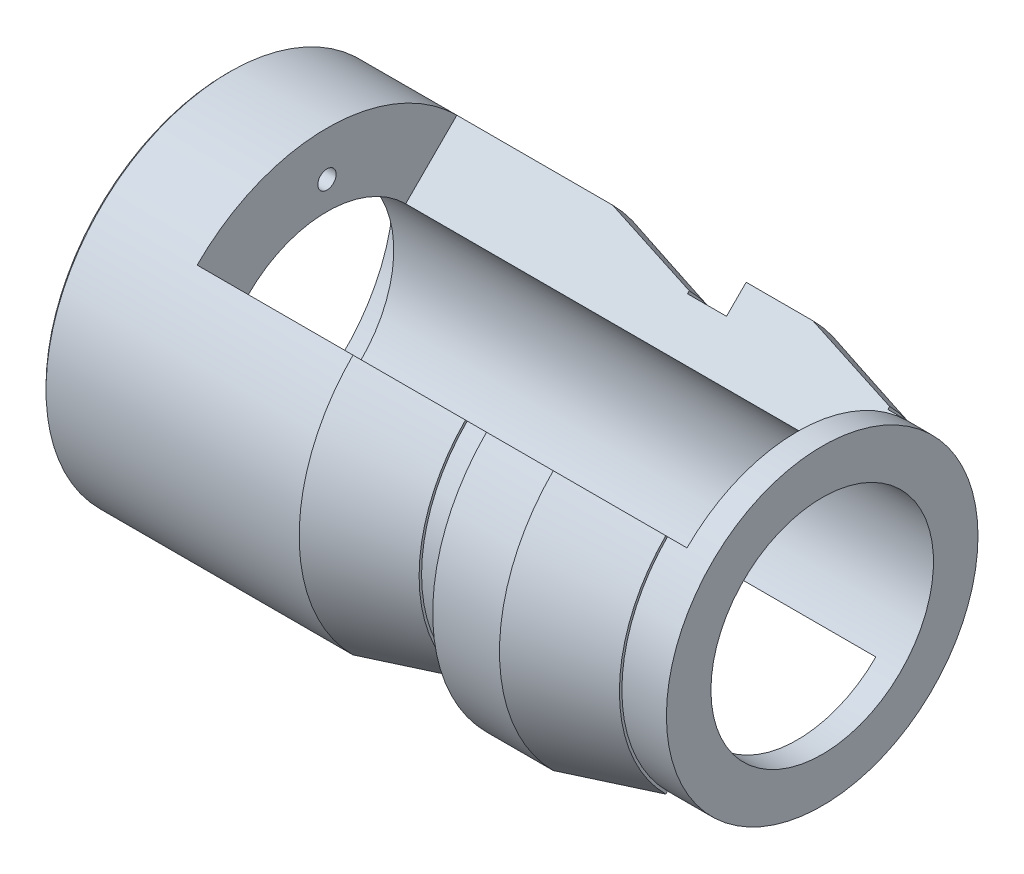
from build123d import *

# Parameters (mm, degrees)
CUT_REVOLVE_1_ANGLE    = 90
CHAMFER_1_SIZE         = 0.5
HOLE_WIZARD_M4_1_D     = 3.3
HOLE_WIZARD_M4_1_DEPTH = 11.5
HOLE_WIZARD_M4_1_TIP   = 0.991420021


with BuildPart() as part:
    # 草图1 → 旋转1 (revolve)
    with BuildSketch(Plane.XY, mode=Mode.PRIVATE) as revolve_1_sk:
        Polygon((0, 30), (10, 30), (10, 20), (107, 20), (107, 28), (99, 28), (99, 28.444863729), (82, 33), (70, 33), (70, 28), (63, 28), (63, 28.444863729), (46, 33), (0, 33), align=None)
    revolve(revolve_1_sk.sketch.rotate(Axis((0, 0, 0), (1, 0, 0)), 90), axis=Axis((0, 0, 0), (1, 0, 0)))

    # 草图2 → 切除-旋转1 (revolve, symmetric, cut)
    with BuildSketch(Plane.XY) as cut_revolve_1_sk:
        Polygon((18, 33), (52.5, 33), (52.5, 38), (102.5, 38), (102.5, 20), (18, 20), align=None)
    cut_revolve_1 = revolve(axis=Axis((0, 0, 0), (1, 0, 0)), revolution_arc=CUT_REVOLVE_1_ANGLE / 2, mode=Mode.SUBTRACT)
    cut_revolve_1 = cut_revolve_1 + revolve(cut_revolve_1_sk.sketch, axis=Axis((0, 0, 0), (-1, 0, 0)), revolution_arc=CUT_REVOLVE_1_ANGLE / 2, mode=Mode.SUBTRACT)

    # 镜向1: 切除-旋转1 across plane
    add(cut_revolve_1.mirror(Plane.ZX), mode=Mode.SUBTRACT)

    # 倒角1
    chamfer_1_edges = [part.edges().sort_by_distance(p)[0] for p in [
        (0, 0, -33),
    ]]
    chamfer(chamfer_1_edges, length=CHAMFER_1_SIZE)

    # M4 螺纹孔1
    with Locations(Plane.ZY.offset(-10)):
        with Locations((0, 25), (25, 0), (0, -25), (-25, 0)):
            Hole(HOLE_WIZARD_M4_1_D / 2, depth=HOLE_WIZARD_M4_1_DEPTH)
            with Locations((0, 0, -(HOLE_WIZARD_M4_1_DEPTH + HOLE_WIZARD_M4_1_TIP / 2))):  # 118° drill point
                Cone(0, HOLE_WIZARD_M4_1_D / 2, HOLE_WIZARD_M4_1_TIP, mode=Mode.SUBTRACT)


solid = part.part
